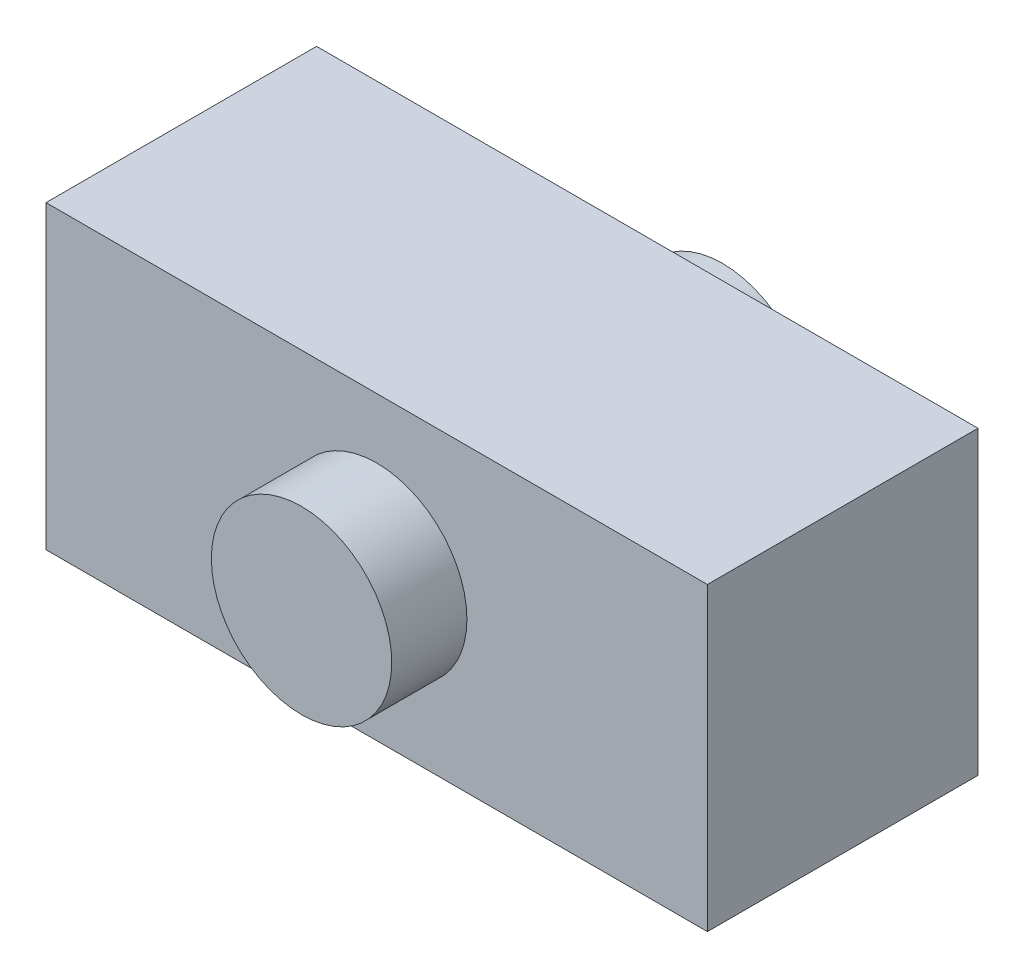
from build123d import *

# Parameters (mm, degrees)
SKETCH_1_W      = 44
SKETCH_1_H      = 20
EXTRUDE_1_DEPTH = 9
SKETCH_2_R      = 6
EXTRUDE_2_DEPTH = 14


with BuildPart() as part:
    # 草图1 → 凸台-拉伸1 (new, symmetric)
    with BuildSketch(Plane.XY):
        Rectangle(SKETCH_1_W, SKETCH_1_H)
    extrude(amount=EXTRUDE_1_DEPTH, both=True)

    # 草图2 → 凸台-拉伸2 (add, symmetric)
    with BuildSketch(Plane.XY):
        Circle(SKETCH_2_R)
    extrude(amount=EXTRUDE_2_DEPTH, both=True)


solid = part.part
